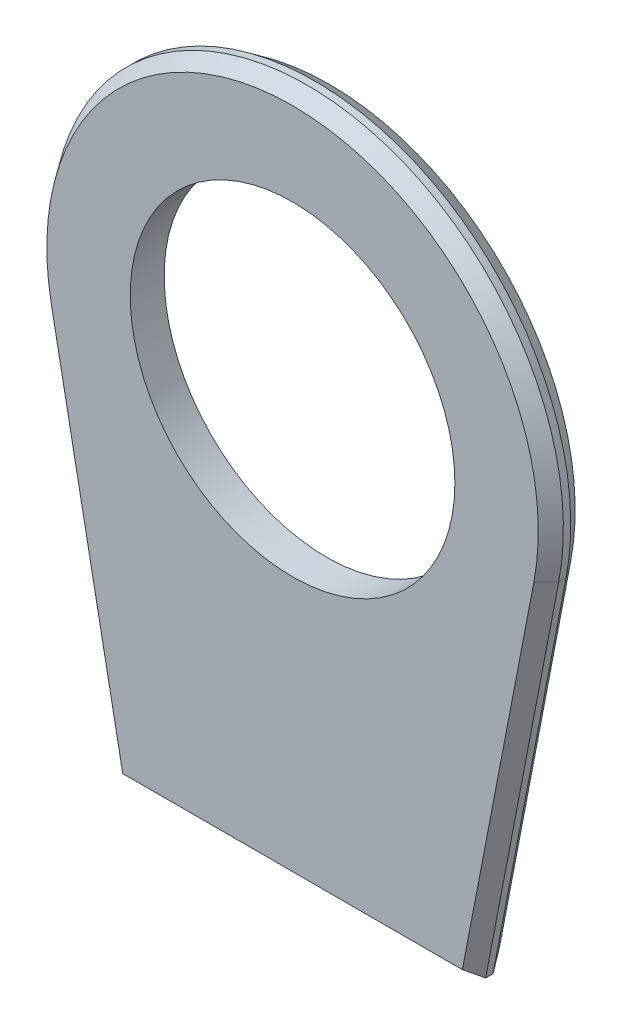
from build123d import *
from OCP.BRepFilletAPI import BRepFilletAPI_MakeChamfer

# Parameters (mm, degrees)
SKETCH1_R           = 110
BOSS_EXTRUDE1_DEPTH = 25
SKETCH2_R           = 123
SKETCH2_R_2         = 110
CUT_EXTRUDE2_DEPTH  = 2
CHAMFER1_SIZE       = 7
CHAMFER1_SIZE2      = 10
CHAMFER2_SIZE       = 10
CHAMFER2_SIZE2      = 7


with BuildPart() as part:
    # Sketch1 → Boss-Extrude1 (new body)
    with BuildSketch(Plane.XY):
        with BuildLine():
            Line((-120.85, 0), (120.85, 0))
            Line((120.85, 0), (170.370762123, 257.196746905))
            ThreePointArc((170.370762123, 257.196746905), (0, 463.5), (-170.370762123, 257.196746905))
            Line((-170.370762123, 257.196746905), (-120.85, 0))
        make_face()
        with Locations((0, 290)):
            Circle(SKETCH1_R, mode=Mode.SUBTRACT)
    extrude(amount=BOSS_EXTRUDE1_DEPTH)

    # Sketch2 → Cut-Extrude2 (cut)
    with BuildSketch(Plane.XY):
        with Locations((0, 290)):
            Circle(SKETCH2_R)
        with Locations((0, 290)):
            Circle(SKETCH2_R_2, mode=Mode.SUBTRACT)
    extrude(amount=CUT_EXTRUDE2_DEPTH, mode=Mode.SUBTRACT)

    # Chamfer1
    chamfer1_edges = [part.edges().sort_by_distance(p)[0] for p in [
        (0, 463.5, 0),
        (145.610381062, 128.598373453, 0),
        (0, 0, 0),
        (-145.610381062, 128.598373453, 0),
    ]]
    chamfer1_side = [part.faces().sort_by_distance(p)[0] for p in [
        (-139.924807111, 129.693076082, 0),
    ]]
    chamfer(chamfer1_edges, length=CHAMFER1_SIZE, length2=CHAMFER1_SIZE2, reference=chamfer1_side[0])

    # Chamfer2: one chamfer whose edges measure the first distance from different faces: ONE call of the kernel's chamfer builder (chamfer() names one face for all edges)
    chamfer2_edges_1 = [part.edges().sort_by_distance(p)[0] for p in [
        (145.610381062, 128.598373453, 25),
    ]]
    chamfer2_side_1 = [part.faces().sort_by_distance(p)[0] for p in [
        (145.610381062, 128.598373453, 17.5),
    ]]
    chamfer2_edges_2 = [part.edges().sort_by_distance(p)[0] for p in [
        (0, 463.5, 25),
    ]]
    chamfer2_side_2 = [part.faces().sort_by_distance(p)[0] for p in [
        (0, 463.5, 17.5),
    ]]
    chamfer2_edges_3 = [part.edges().sort_by_distance(p)[0] for p in [
        (-145.610381062, 128.598373453, 25),
    ]]
    chamfer2_side_3 = [part.faces().sort_by_distance(p)[0] for p in [
        (-145.610381062, 128.598373453, 17.5),
    ]]
    chamfer2_edges_4 = [part.edges().sort_by_distance(p)[0] for p in [
        (0, 0, 25),
    ]]
    chamfer2_side_4 = [part.faces().sort_by_distance(p)[0] for p in [
        (0, 0, 17.5),
    ]]
    chamfer2 = BRepFilletAPI_MakeChamfer(part.part.solid().wrapped)
    for e in chamfer2_edges_1:
        chamfer2.Add(CHAMFER2_SIZE, CHAMFER2_SIZE2, e.wrapped, chamfer2_side_1[0].wrapped)  # the first distance lies on this face
    for e in chamfer2_edges_2:
        chamfer2.Add(CHAMFER2_SIZE, CHAMFER2_SIZE2, e.wrapped, chamfer2_side_2[0].wrapped)  # the first distance lies on this face
    for e in chamfer2_edges_3:
        chamfer2.Add(CHAMFER2_SIZE, CHAMFER2_SIZE2, e.wrapped, chamfer2_side_3[0].wrapped)  # the first distance lies on this face
    for e in chamfer2_edges_4:
        chamfer2.Add(CHAMFER2_SIZE, CHAMFER2_SIZE2, e.wrapped, chamfer2_side_4[0].wrapped)  # the first distance lies on this face
    add(Compound.cast(chamfer2.Shape()), mode=Mode.REPLACE)


solid = part.part
